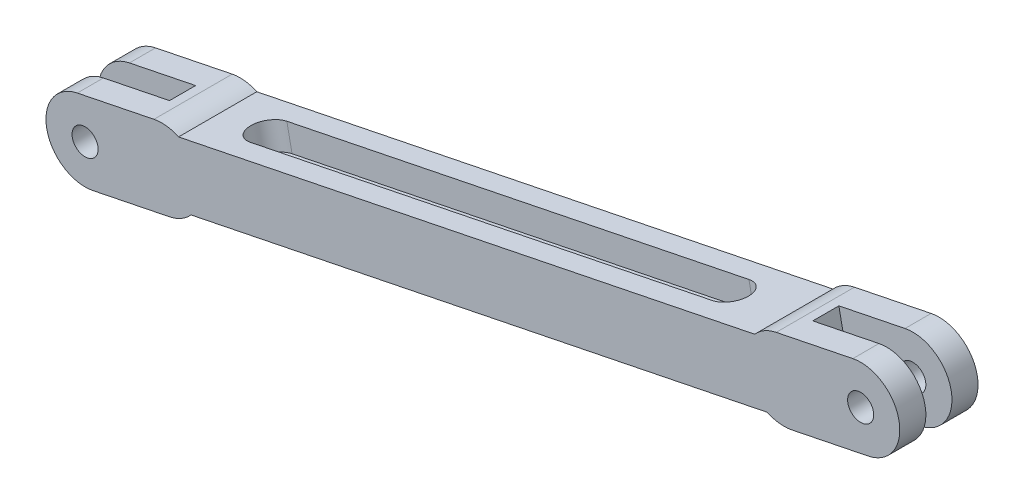
SolidWorks part; units mm, degrees
ref_plane "Front Plane" through (0, 0, 0) normal (0, 0, 1) x (1, 0, 0)
ref_plane "Top Plane" through (0, 0, 0) normal (0, 1, 0) x (1, 0, 0)
ref_plane "Right Plane" through (0, 0, 0) normal (1, 0, 0) x (0, 0, -1)
sketch "Sketch1" plane through (0, 0, 3001.3357) normal (0, 0, 1) x (1, 0, 0)
  line L6 (917.9349, 337.7344) -> (888.5372, 331.7533)
  line L7 (880.316, 327.0192) -> (659.4068, 282.0741)
  line L8 (649.9894, 283.2195) -> (620.5916, 277.2384)
  line L9 (626.5728, 247.8407) -> (655.9705, 253.8218)
  line L10 (664.1917, 258.5559) -> (885.1009, 303.501)
  line L11 (894.5183, 302.3556) -> (923.916, 308.3367)
  line L12 (917.9349, 337.7344) -> (888.5372, 331.7533)
  line L13 (880.316, 327.0192) -> (659.4068, 282.0741)
  line L14 (649.9894, 283.2195) -> (620.5916, 277.2384)
  line L15 (626.5728, 247.8407) -> (655.9705, 253.8218)
  line L16 (664.1917, 258.5559) -> (885.1009, 303.501)
  line L17 (894.5183, 302.3556) -> (923.916, 308.3367)
  arc A0 (618.6826, 261.5427) -> (628.4818, 263.5364) centre (623.5822, 262.5395) ccw construction
  arc A1 (628.4818, 263.5364) -> (618.6826, 261.5427) centre (623.5822, 262.5395) ccw construction
  arc A2 (618.6826, 261.5427) -> (628.4818, 263.5364) centre (623.5822, 262.5395) ccw
  arc A3 (628.4818, 263.5364) -> (618.6826, 261.5427) centre (623.5822, 262.5395) ccw
  arc A4 (916.0259, 322.0387) -> (925.8251, 324.0324) centre (920.9255, 323.0356) ccw construction
  arc A5 (925.8251, 324.0324) -> (916.0259, 322.0387) centre (920.9255, 323.0356) ccw construction
  arc A6 (923.916, 308.3367) -> (917.9349, 337.7344) centre (920.9255, 323.0356) ccw
  arc A7 (888.5372, 331.7533) -> (880.316, 327.0192) centre (891.5278, 317.0544) ccw
  arc A8 (659.4068, 282.0741) -> (649.9894, 283.2195) centre (652.9799, 268.5207) ccw
  arc A9 (620.5916, 277.2384) -> (626.5728, 247.8407) centre (623.5822, 262.5395) ccw
  arc A10 (655.9705, 253.8218) -> (664.1917, 258.5559) centre (652.9799, 268.5207) ccw
  arc A11 (885.1009, 303.501) -> (894.5183, 302.3556) centre (891.5278, 317.0544) ccw
  arc A12 (923.916, 308.3367) -> (917.9349, 337.7344) centre (920.9255, 323.0356) ccw
  arc A13 (888.5372, 331.7533) -> (880.316, 327.0192) centre (891.5278, 317.0544) ccw
  arc A14 (659.4068, 282.0741) -> (649.9894, 283.2195) centre (652.9799, 268.5207) ccw
  arc A15 (620.5916, 277.2384) -> (626.5728, 247.8407) centre (623.5822, 262.5395) ccw
  arc A16 (655.9705, 253.8218) -> (664.1917, 258.5559) centre (652.9799, 268.5207) ccw
  arc A17 (885.1009, 303.501) -> (894.5183, 302.3556) centre (891.5278, 317.0544) ccw
  arc A18 (916.0259, 322.0387) -> (925.8251, 324.0324) centre (920.9255, 323.0356) ccw
  arc A19 (925.8251, 324.0324) -> (916.0259, 322.0387) centre (920.9255, 323.0356) ccw
  dimension "D1" = 0
extrude "Boss-Extrude1" add sketch "Sketch1" against normal up to surface (30 mm away)
sketch "Sketch2" plane through (-23.5147, 115.577, 0) normal (0.1994, -0.9799, 0) x (0.9799, 0.1994, 0)
  line L0 (981.8409, 3001.3357) -> (966.8409, 3001.3357) construction
  line L1 (940.9557, 2991.3357) -> (986.7704, 2991.3357)
  line L2 (940.9557, 2991.3357) -> (940.9557, 2981.3357)
  line L3 (940.9557, 2981.3357) -> (986.7704, 2981.3357)
  line L4 (986.7704, 2991.3357) -> (986.7704, 2981.3357)
  line L5 (940.9557, 2991.3357) -> (986.7704, 2981.3357) construction
  line L6 (940.9557, 2981.3357) -> (986.7704, 2991.3357) construction
  line L8 (815.1234, 2937.3272) -> (815.1234, 3041.3812) construction
  line L9 (702.4059, 3001.3357) -> (927.8409, 3001.3357) construction
  line L10 (689.2911, 2981.3357) -> (643.4764, 2991.3357) construction
  line L11 (689.2911, 2991.3357) -> (643.4764, 2981.3357) construction
  line L12 (643.4764, 2991.3357) -> (643.4764, 2981.3357)
  line L13 (689.2911, 2981.3357) -> (643.4764, 2981.3357)
  line L14 (689.2911, 2991.3357) -> (689.2911, 2981.3357)
  line L15 (689.2911, 2991.3357) -> (643.4764, 2991.3357)
  point P0 (963.8631, 2986.3357)
  point P11 (815.1234, 3001.3357)
  point P16 (666.3838, 2986.3357)
  dimension "D1" = 10
  dimension "D2" = 10
extrude "Cut-Extrude1" cut sketch "Sketch2" against normal blind 80
sketch "Sketch3" plane through (-24.1129, 118.5168, 0) normal (0.1994, -0.9799, 0) x (0.9799, 0.1994, 0)
  line L0 (722.3379, 2986.3357) -> (903.12, 2986.3357) construction
  line L1 (722.3379, 2993.3357) -> (903.12, 2993.3357)
  line L2 (722.3379, 2979.3357) -> (903.12, 2979.3357)
  line L3 (927.8409, 2971.3357) -> (702.4059, 2971.3357) construction
  arc A0 (722.3379, 2993.3357) -> (722.3379, 2979.3357) centre (722.3379, 2986.3357) ccw
  arc A1 (903.12, 2979.3357) -> (903.12, 2993.3357) centre (903.12, 2986.3357) ccw
  point P2 (812.729, 2986.3357)
  dimension "D1" = 7
  dimension "D2" = 8
extrude "Cut-Extrude2" cut sketch "Sketch3" against normal blind 10
ref_plane "Plane1" through (-26.5053, 130.2759, 0) normal (0.1994, -0.9799, 0) x (-0.9799, -0.1994, 0)
mirror "Mirror1" about plane through (-26.5053, 130.2759, 0) normal (0.1994, -0.9799, 0) of "Cut-Extrude2"
